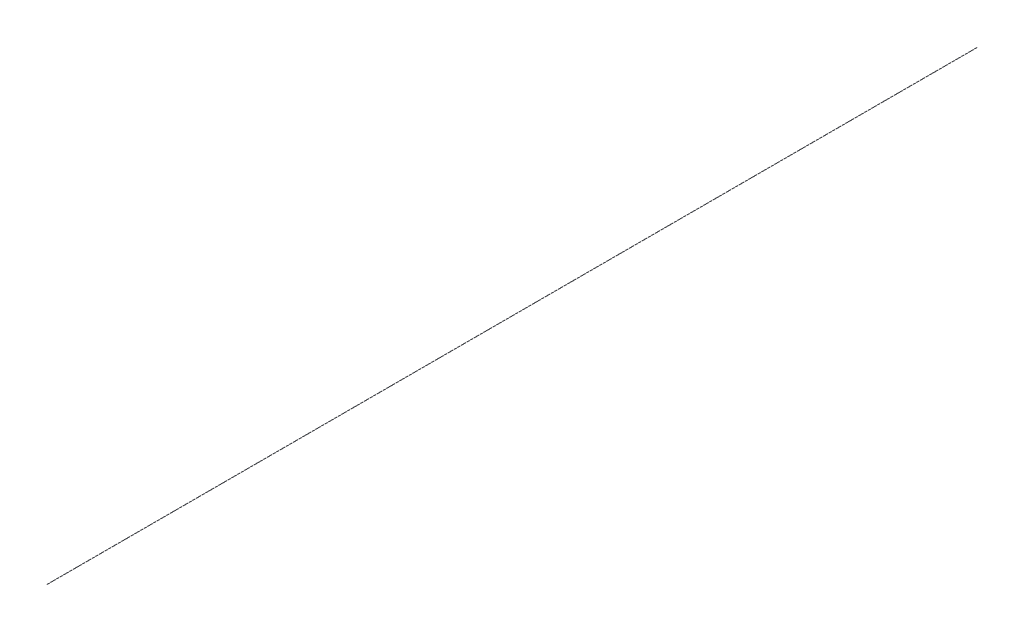
SolidWorks part; units mm, degrees
ref_plane "Front Plane" through (0, 0, 0) normal (0, 0, 1) x (1, 0, 0)
ref_plane "Top Plane" through (0, 0, 0) normal (0, 1, 0) x (1, 0, 0)
ref_plane "Right Plane" through (0, 0, 0) normal (1, 0, 0) x (0, 0, -1)
sketch "Sketch1" plane through (0, 0, 0) normal (0, 0, 1) x (1, 0, 0)
  circle A0 centre (0, 0) radius 0.075
  circle A1 centre (0, 0) radius 0.15
  dimension "D1" = 0.15
  dimension "D2" = 0.3
extrude "Boss-Extrude1" add sketch "Sketch1" along normal blind 1900
